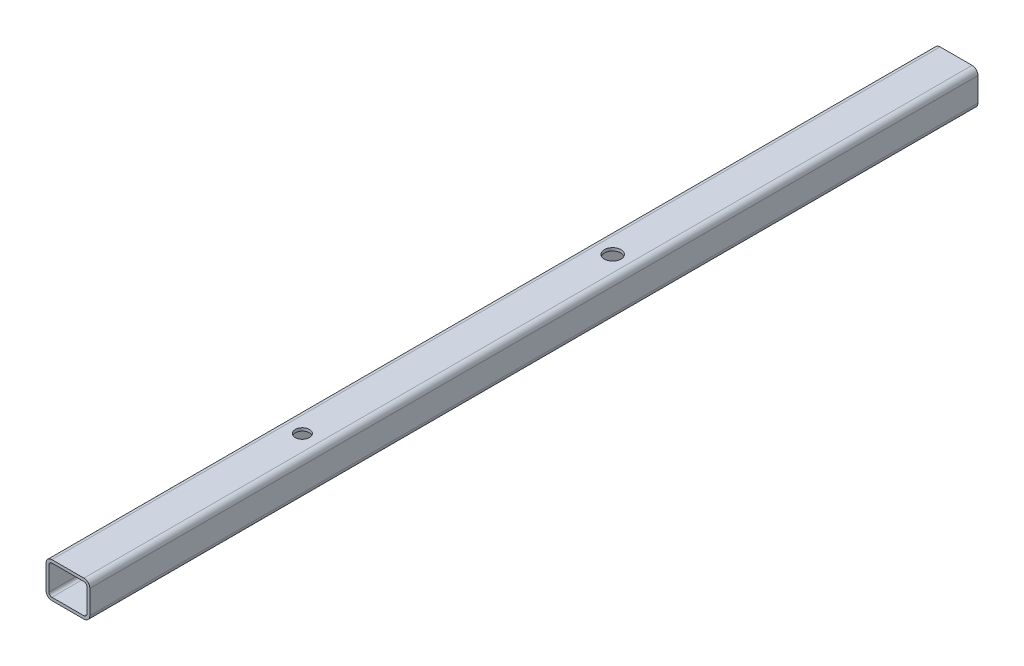
from build123d import *

# Parameters (mm, degrees)
EXTRUDE_1_DEPTH          = 200
EXTRUDE_1_DEPTH_BACK     = 300
SKETCH_7_R               = 6
CUT_EXTRUDE_2_DEPTH      = 83
CUT_EXTRUDE_3_DEPTH      = 303.063321176
CUT_EXTRUDE_3_DEPTH_BACK = 303.063321176
SKETCH_8_R               = 7
EXTRUDE_START            = 250
EXTRUDE_4_DEPTH          = 250


with BuildPart() as part:
    # Sketch 205 → 凸台-拉伸1 (new, two sides: drawn at the far end of the back side and taken through both)
    with BuildSketch(Plane.XY.offset(-EXTRUDE_1_DEPTH_BACK)):
        with BuildLine():
            Line((-13.5, 15), (13.5, 15))
            ThreePointArc((13.5, 15), (17.035533906, 13.535533906), (18.5, 10))
            Line((18.5, 10), (18.5, -10))
            ThreePointArc((18.5, -10), (17.035533906, -13.535533906), (13.5, -15))
            Line((13.5, -15), (-13.5, -15))
            ThreePointArc((-13.5, -15), (-17.035533906, -13.535533906), (-18.5, -10))
            Line((-18.5, -10), (-18.5, 10))
            ThreePointArc((-18.5, 10), (-17.035533906, 13.535533906), (-13.5, 15))
        make_face()
        with BuildLine():
            Line((-13.5, 12.5), (13.5, 12.5))
            ThreePointArc((13.5, 12.5), (15.267766953, 11.767766953), (16, 10))
            Line((16, 10), (16, -10))
            ThreePointArc((16, -10), (15.267766953, -11.767766953), (13.5, -12.5))
            Line((13.5, -12.5), (-13.5, -12.5))
            ThreePointArc((-13.5, -12.5), (-15.267766953, -11.767766953), (-16, -10))
            Line((-16, -10), (-16, 10))
            ThreePointArc((-16, 10), (-15.267766953, 11.767766953), (-13.5, 12.5))
        make_face(mode=Mode.SUBTRACT)
    extrude(amount=EXTRUDE_1_DEPTH + EXTRUDE_1_DEPTH_BACK)

    # 草图7 → 切除-拉伸2 (cut)
    with BuildSketch(Plane(origin=(0, 15, 0), x_dir=(1, 0, 0), z_dir=(0, 1, 0))):
        with Locations((0, -2)):
            Circle(SKETCH_7_R)
    extrude(amount=-CUT_EXTRUDE_2_DEPTH, mode=Mode.SUBTRACT)

    # 草图8 → 切除-拉伸3 (cut, two sides: drawn at the far end of the back side and taken through both)
    with BuildSketch(Plane(origin=(0, 15, 0), x_dir=(1, 0, 0), z_dir=(0, 1, 0)).offset(-CUT_EXTRUDE_3_DEPTH_BACK)):
        with Locations(Location((0, 260, 0), (0, 0, 180))):
            Circle(SKETCH_8_R)
    extrude(amount=CUT_EXTRUDE_3_DEPTH + CUT_EXTRUDE_3_DEPTH_BACK, mode=Mode.SUBTRACT)

    # 草图11 → 凸台-拉伸4 (add)
    with BuildSketch(Plane(origin=(0, 0, -300), x_dir=(-1, 0, 0), z_dir=(0, 0, -1)).offset(EXTRUDE_START)):
        with BuildLine():
            Line((18.5, -10), (18.5, 10))
            ThreePointArc((18.5, 10), (17.035533906, 13.535533906), (13.5, 15))
            Line((13.5, 15), (-13.5, 15))
            ThreePointArc((-13.5, 15), (-17.035533906, 13.535533906), (-18.5, 10))
            Line((-18.5, 10), (-18.5, -10))
            ThreePointArc((-18.5, -10), (-17.035533906, -13.535533906), (-13.5, -15))
            Line((-13.5, -15), (13.5, -15))
            ThreePointArc((13.5, -15), (17.035533906, -13.535533906), (18.5, -10))
        make_face()
        with BuildLine():
            Line((-16, -12.5), (13.5, -12.5))
            ThreePointArc((13.5, -12.5), (15.267766953, -11.767766953), (16, -10))
            Line((16, -10), (16, 10))
            ThreePointArc((16, 10), (15.267766953, 11.767766953), (13.5, 12.5))
            Line((13.5, 12.5), (-13.5, 12.5))
            ThreePointArc((-13.5, 12.5), (-15.267766953, 11.767766953), (-16, 10))
            Line((-16, 10), (-16, -12.5))
        make_face(mode=Mode.SUBTRACT)
    extrude(amount=-EXTRUDE_4_DEPTH)


solid = part.part
